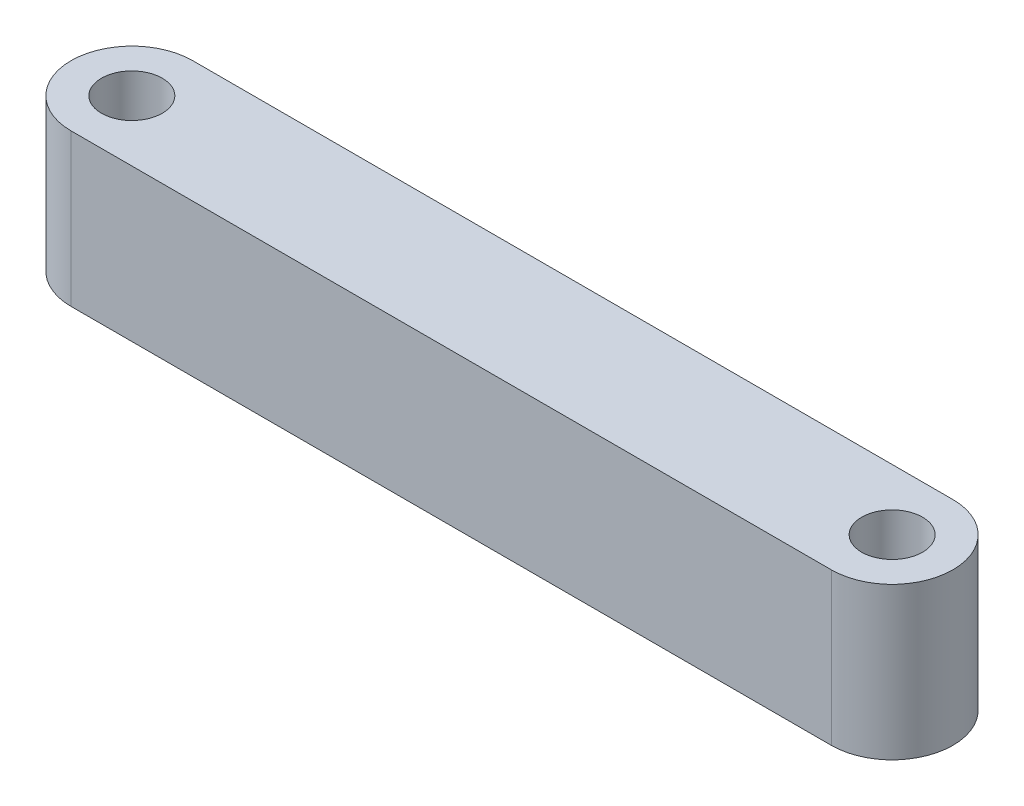
from build123d import *

# Parameters (mm, degrees)
SKETCH1_R           = 2
BOSS_EXTRUDE1_DEPTH = 10


with BuildPart() as part:
    # Sketch1 → Boss-Extrude1 (new body)
    with BuildSketch(Plane(origin=(0, 0, 0), x_dir=(1, 0, 0), z_dir=(0, 1, 0))):
        with BuildLine():
            Line((-25, 4), (25, 4))
            ThreePointArc((25, 4), (29, 0), (25, -4))
            Line((25, -4), (-25, -4))
            ThreePointArc((-25, -4), (-29, 0), (-25, 4))
        make_face()
        with Locations(Location((-25, 0, 0), (0, 0, 270))):
            Circle(SKETCH1_R, mode=Mode.SUBTRACT)
        with Locations(Location((25, 0, 0), (0, 0, 270))):
            Circle(SKETCH1_R, mode=Mode.SUBTRACT)
    extrude(amount=BOSS_EXTRUDE1_DEPTH)


solid = part.part
